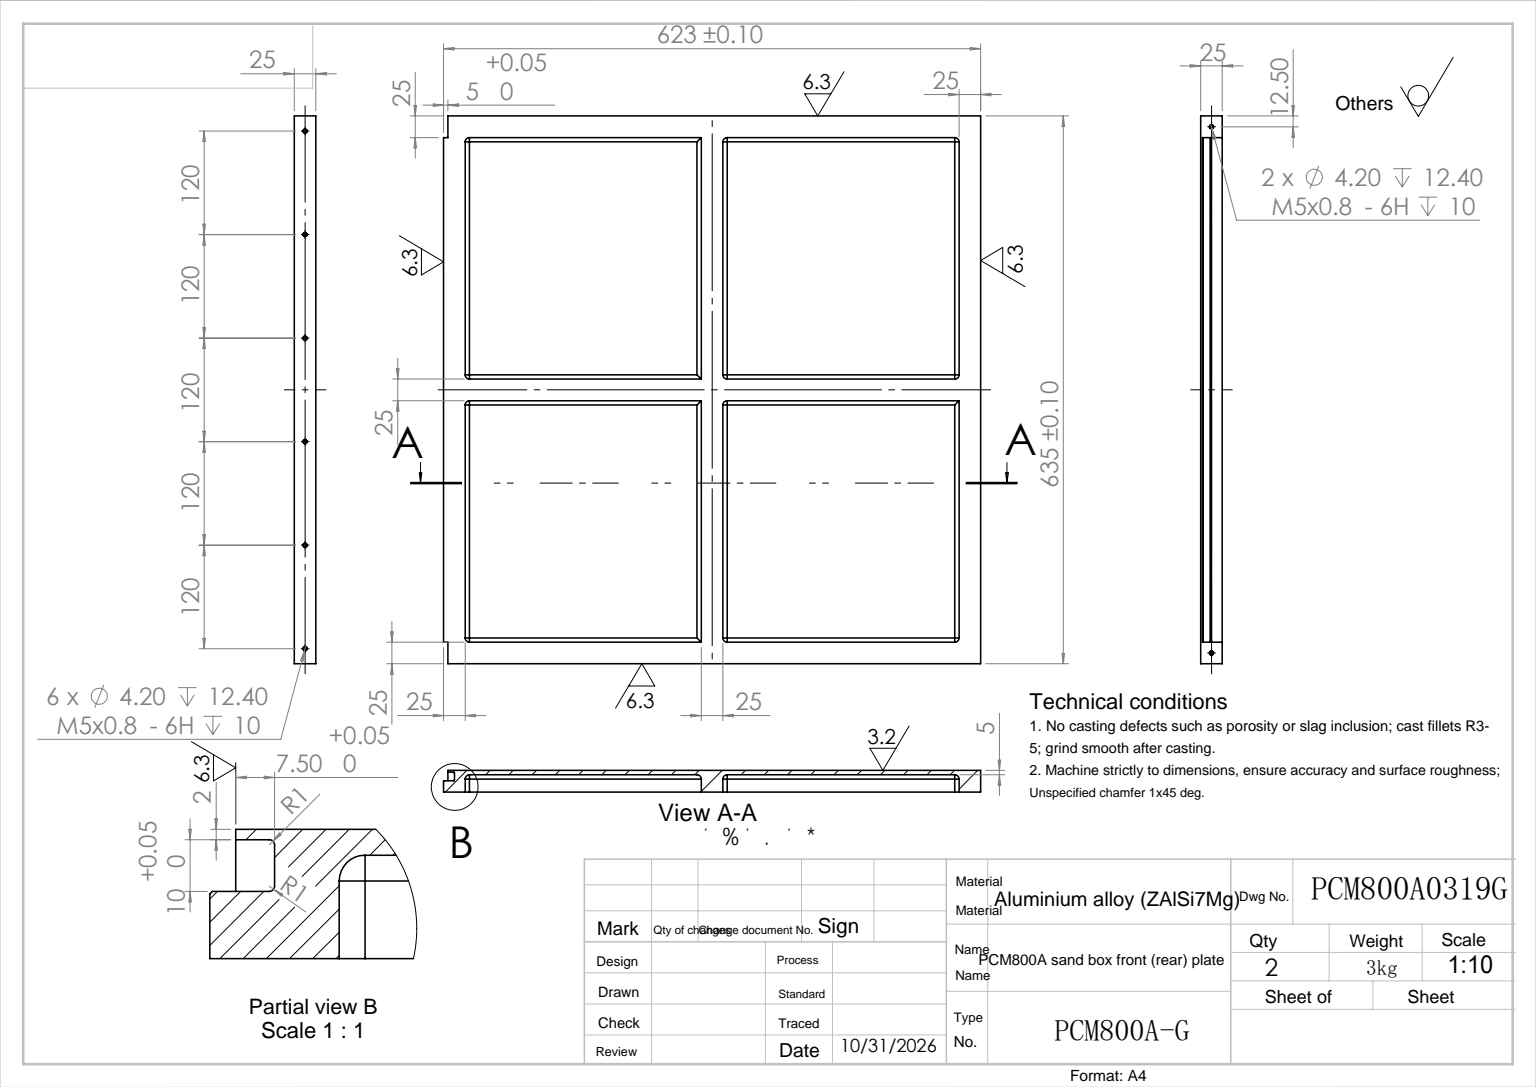
SolidWorks part; units mm, degrees
ref_plane "前视" through (0, 0, 0) normal (0, 0, 1) x (1, 0, 0)
ref_plane "上视" through (0, 0, 0) normal (0, 1, 0) x (1, 0, 0)
ref_plane "右视" through (0, 0, 0) normal (1, 0, 0) x (0, 0, -1)
sketch "草图1" plane through (0, 0, 0) normal (0, 0, 1) x (1, 0, 0)
  line L1 (0, 0) -> (623, 0)
  line L2 (0, 0) -> (0, 635)
  line L3 (0, 635) -> (623, 635)
  line L4 (623, 0) -> (623, 635)
  dimension "D1" = 635
  dimension "D2" = 623
extrude "拉伸1" add sketch "草图1" along normal blind 5
sketch "草图2" plane through (0, 0, 5) normal (0, 0, 1) x (1, 0, 0)
  line L0 (0, 0) -> (623, 0) construction
  line L1 (0, 635) -> (25, 635)
  line L2 (0, 635) -> (0, 0)
  line L3 (0, 0) -> (25, 0)
  line L4 (25, 635) -> (25, 0)
  dimension "D1" = 25
extrude "拉伸2" add sketch "草图2" along normal blind 20
sketch "草图3" plane through (0, 0, 5) normal (0, 0, 1) x (1, 0, 0)
  line L0 (25, 0) -> (623, 0) construction
  line L1 (623, 635) -> (598, 635)
  line L2 (623, 635) -> (623, 0)
  line L3 (623, 0) -> (598, 0)
  line L4 (598, 635) -> (598, 0)
  dimension "D1" = 25
extrude "拉伸3" add sketch "草图3" along normal blind 20
sketch "草图4" plane through (0, 635, 0) normal (0, 1, 0) x (-1, 0, 0)
  line L0 (0, 0) -> (-5, 0)
  line L1 (-623, 0) -> (0, 0) construction
  line L2 (-5, 0) -> (-5, 2)
  line L3 (-5, 2) -> (-11.5, 2)
  line L4 (-12.5, 3) -> (-12.5, 11)
  line L5 (-11.5, 12) -> (0, 12)
  line L7 (0, 0) -> (0, 12)
  arc A0 (-11.5, 2) -> (-12.5, 3) centre (-11.5, 3) cw
  arc A1 (-11.5, 12) -> (-12.5, 11) centre (-11.5, 11) ccw
  point P14 (-12.5, 2)
  point P17 (-12.5, 12)
  dimension "D5" = 1
  dimension "D1" = 5
  dimension "D2" = 2
  dimension "D3" = 7.5
  dimension "D4" = 10
extrude "切除-拉伸1" cut sketch "草图4" against normal through all
chamfer "倒角1" distance 0.5 angle 45 1 edges at (0, 317.5, 12)
sketch "草图7" plane through (0, 0, 5) normal (0, 0, 1) x (1, 0, 0)
  line L0 (598, 635) -> (598, 0) construction
  line L1 (25, 635) -> (598, 635)
  line L2 (25, 635) -> (25, 610)
  line L3 (25, 610) -> (598, 610)
  line L4 (598, 635) -> (598, 610)
  dimension "D1" = 25
extrude "拉伸4" add sketch "草图7" along normal blind 20
sketch "草图8" plane through (0, 0, 5) normal (0, 0, 1) x (1, 0, 0)
  line L0 (598, 610) -> (598, 0) construction
  line L1 (25, 0) -> (598, 0)
  line L2 (25, 0) -> (25, 25)
  line L3 (25, 25) -> (598, 25)
  line L4 (598, 0) -> (598, 25)
  dimension "D1" = 25
extrude "拉伸5" add sketch "草图8" along normal blind 20
sketch "草图9" plane through (0, 0, 5) normal (0, 0, 1) x (1, 0, 0)
  line L0 (25, 25) -> (25, 610) construction
  line L1 (25, 330) -> (598, 330)
  line L2 (25, 330) -> (25, 305)
  line L3 (25, 305) -> (598, 305)
  line L4 (598, 330) -> (598, 305)
  line L5 (598, 610) -> (598, 25) construction
  line L6 (598, 25) -> (25, 25) construction
  dimension "D1" = 25
  dimension "D2" = 280
extrude "拉伸6" add sketch "草图9" along normal blind 20
sketch "草图10" plane through (0, 0, 5) normal (0, 0, 1) x (1, 0, 0)
  line L0 (25, 610) -> (598, 610) construction
  line L1 (299, 610) -> (324, 610)
  line L2 (299, 610) -> (299, 25)
  line L3 (299, 25) -> (324, 25)
  line L4 (324, 610) -> (324, 25)
  line L5 (598, 25) -> (25, 25) construction
  line L6 (25, 330) -> (25, 610) construction
  dimension "D1" = 25
  dimension "D2" = 274
extrude "拉伸7" add sketch "草图10" along normal blind 20
sketch "草图11" plane through (0, 635, 0) normal (0, 1, 0) x (-1, 0, 0)
  line L0 (-5, 2) -> (-5, 12)
  line L1 (-0.5, 12) -> (-11.5, 12) construction
  line L2 (-5, 12) -> (-11.5, 12)
  line L3 (-12.5, 11) -> (-12.5, 3)
  line L4 (-11.5, 2) -> (-5, 2)
  arc A0 (-11.5, 2) -> (-12.5, 3) centre (-11.5, 3) cw
  arc A1 (-11.5, 12) -> (-12.5, 11) centre (-11.5, 11) ccw
  point P12 (-12.5, 12)
  dimension "D1" = 1
  dimension "D3" = 1
  dimension "D2" = 7.5
extrude "拉伸8" add sketch "草图11" against normal blind 25
sketch "草图12" plane through (0, 635, 0) normal (0, 1, 0) x (-1, 0, 0)
  line L0 (-5, 12) -> (-0.5, 12)
  line L1 (-0.5, 12) -> (0, 12.5)
  line L2 (0, 12.5) -> (0, 25)
  line L3 (0, 25) -> (-5, 25)
  line L4 (-623, 25) -> (0, 25) construction
  line L5 (-5, 25) -> (-5, 12)
extrude "切除-拉伸2" cut sketch "草图12" against normal blind 25
sketch "草图13" plane through (0, 0, 0) normal (0, -1, 0) x (1, 0, 0)
  line L0 (5, 2) -> (5, 12)
  line L1 (5, 12) -> (11.5, 12)
  line L2 (12.5, 11) -> (12.5, 3)
  line L3 (11.5, 2) -> (5, 2)
  arc A0 (11.5, 2) -> (12.5, 3) centre (11.5, 3) ccw
  arc A1 (11.5, 12) -> (12.5, 11) centre (11.5, 11) cw
  dimension "D1" = 1
extrude "拉伸9" add sketch "草图13" against normal blind 25
sketch "草图14" plane through (0, 0, 0) normal (0, -1, 0) x (1, 0, 0)
  line L0 (5, 12) -> (5, 25)
  line L1 (5, 25) -> (0, 25)
  line L2 (0, 25) -> (0, 12.5)
  line L3 (0, 12.5) -> (0.5, 12)
  line L4 (0.5, 12) -> (5, 12)
extrude "切除-拉伸3" cut sketch "草图14" against normal blind 25
sketch "草图15" plane through (623, 0, 0) normal (1, 0, 0) x (0, 0, -1)
  line L0 (-12.5, 635) -> (-12.5, 0) construction
  line L1 (-25, 635) -> (0, 635) construction
  line L2 (-25, 0) -> (0, 0) construction
  line L3 (-12.5, 617.5) -> (0, 617.5) construction
  line L4 (0, 0) -> (0, 635) construction
  line L5 (-12.5, 497.5) -> (0, 497.5) construction
  line L6 (-12.5, 377.5) -> (0, 377.5) construction
  line L7 (-12.5, 257.5) -> (0, 257.5) construction
  line L8 (-12.5, 137.5) -> (0, 137.5) construction
  line L9 (-12.5, 17.5) -> (0, 17.5) construction
  dimension "D1" = 17.5
  dimension "D2" = 120
hole_wizard "M5x0.8 螺纹孔1" positions "3D草图1" profile "草图16" tap size "M5x0.8" standard "Ansi Metric"
sketch3d "3D草图1"
  point P0 (623, 617.5, 12.5)
  point P3 (623, 497.5, 12.5)
  point P6 (623, 377.5, 12.5)
  point P9 (623, 257.5, 12.5)
  point P12 (623, 137.5, 12.5)
  point P15 (623, 17.5, 12.5)
sketch "草图16" plane through (623, 617.5, 12.5) normal (0, 1, 0) x (0, 0, -1)
  line L0 (0, 0) -> (0, 13.6618)
  line L1 (0, 13.6618) -> (2.1, 12.4)
  line L2 (2.1, 12.4) -> (2.1, 10)
  line L3 (2.1, 10) -> (2.5, 10)
  line L4 (2.5, 10) -> (2.5, 0)
  line L5 (2.5, 0) -> (0, 0)
  line L10 (0, 13.6618) -> (-2.1, 12.4) construction
  line L11 (0, -6.35) -> (0, 107.95) construction
  dimension "蹟恇謂郰芛眻噤" = 4.2
  dimension "蹟恇謂郰芛旮僅" = 12.4
  dimension "蹟恇翋眻噤" = 5
  dimension "蹟恇旮僅" = 10
  dimension "絳芛褒僅" = 118
sketch "草图17" plane through (5, 0, 0) normal (-1, 0, 0) x (0, 0, 1)
  line L0 (12.5, 635) -> (12.5, 610) construction
  line L1 (12.5, 622.5) -> (25, 622.5) construction
  line L2 (25, 610) -> (25, 635) construction
  line L3 (12.5, 0) -> (12.5, 25) construction
  line L4 (25, 12.5) -> (12.5, 12.5) construction
  line L5 (25, 25) -> (25, 0) construction
hole_wizard "M5x0.8 螺纹孔2" positions "3D草图2" profile "草图18" tap size "M5x0.8" standard "Ansi Metric"
sketch3d "3D草图2"
  point P0 (5, 12.5, 12.5)
  point P3 (5, 622.5, 12.5)
sketch "草图18" plane through (5, 12.5, 12.5) normal (0, 1, 0) x (0, 0, 1)
  line L0 (0, 0) -> (0, 13.6618)
  line L1 (0, 13.6618) -> (2.1, 12.4)
  line L2 (2.1, 12.4) -> (2.1, 10)
  line L3 (2.1, 10) -> (2.5, 10)
  line L4 (2.5, 10) -> (2.5, 0)
  line L5 (2.5, 0) -> (0, 0)
  line L10 (0, 13.6618) -> (-2.1, 12.4) construction
  line L11 (0, -6.35) -> (0, 107.95) construction
  dimension "蹟恇謂郰芛眻噤" = 4.2
  dimension "蹟恇謂郰芛旮僅" = 12.4
  dimension "蹟恇翋眻噤" = 5
  dimension "蹟恇旮僅" = 10
  dimension "絳芛褒僅" = 118
fillet "圆角1" radius 5 27 edges at (461, 610, 5) (598, 470, 5) (461, 330, 5) (324, 470, 5) (162, 330, 5) (162, 610, 5) (299, 470, 5) (162, 25, 5) (162, 305, 5) (299, 165, 5) (461, 305, 5) (598, 165, 5) (461, 25, 5) (324, 165, 5) (598, 610, 15) (598, 330, 15) (598, 25, 15) (324, 25, 15) (324, 330, 15) (25, 330, 15) (25, 25, 15) (25, 305, 15) (324, 305, 15) (324, 610, 15) (25, 610, 15)
